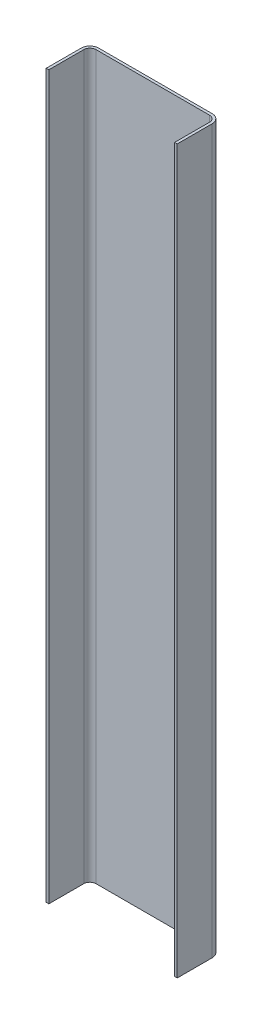
from build123d import *

# Parameters (mm, degrees)
EXTRUDE_THIN1_DEPTH = 413.5


with BuildPart() as part:
    # Sketch1 → Extrude-Thin1 (new, symmetric)
    with BuildSketch(Plane(origin=(0, 0, 0), x_dir=(1, 0, 0), z_dir=(0, 1, 0))):
        with BuildLine():
            Line((-75, -25), (-75, 15))
            ThreePointArc((-75, 15), (-72.071067812, 22.071067812), (-65, 25))
            Line((-65, 25), (65, 25))
            ThreePointArc((65, 25), (72.071067812, 22.071067812), (75, 15))
            Line((75, 15), (75, -25))
            Line((75, -25), (72, -25))
            Line((72, -25), (72, 15))
            ThreePointArc((72, 15), (69.949747468, 19.949747468), (65, 22))
            Line((65, 22), (-65, 22))
            ThreePointArc((-65, 22), (-69.949747468, 19.949747468), (-72, 15))
            Line((-72, 15), (-72, -25))
            Line((-72, -25), (-75, -25))
        make_face()
    extrude(amount=EXTRUDE_THIN1_DEPTH, both=True)


solid = part.part
